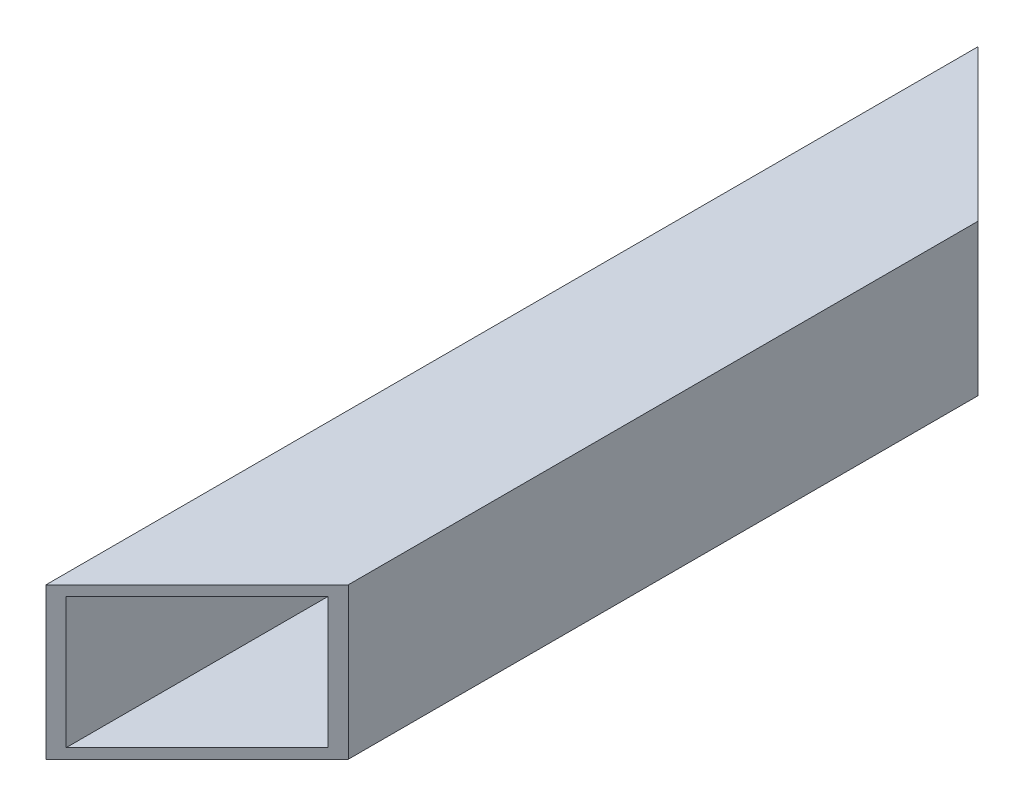
SolidWorks part; units mm, degrees
ref_plane "前视基准面" through (0, 0, 0) normal (0, 0, 1) x (1, 0, 0)
ref_plane "上视基准面" through (0, 0, 0) normal (0, 1, 0) x (1, 0, 0)
ref_plane "右视基准面" through (0, 0, 0) normal (1, 0, 0) x (0, 0, -1)
sketch "草图1" plane through (0, 0, 0) normal (0, 0, 1) x (1, 0, 0)
  line L0 (13, 13) -> (-13, 13)
  line L1 (15, -15) -> (-15, -15)
  line L2 (15, -15) -> (15, 15)
  line L3 (15, 15) -> (-15, 15)
  line L4 (-15, -15) -> (-15, 15)
  line L5 (15, -15) -> (-15, 15) construction
  line L6 (15, 15) -> (-15, -15) construction
  line L7 (-13, -13) -> (-13, 13)
  line L8 (13, -13) -> (-13, -13)
  line L9 (13, -13) -> (13, 13)
  point P0 (0, 0)
  dimension "D1" = 30
  dimension "D2" = 2
extrude "凸台-拉伸1" add sketch "草图1" along normal mid plane 185
sketch "草图2" plane through (0, 15, 0) normal (0, 1, 0) x (1, 0, 0)
  line L0 (-15, 92.5) -> (15, 62.5)
  line L1 (15, -92.5) -> (15, 92.5) construction
  line L2 (15, -62.5) -> (-15, -92.5)
  line L3 (-15, -92.5) -> (-15, 92.5) construction
  line L8 (15, 92.5) -> (-15, 92.5)
  line L9 (-15, 92.5) -> (-15, -92.5)
  line L10 (-15, -92.5) -> (15, -92.5)
  line L11 (15, -92.5) -> (15, 92.5)
  line L12 (15, 92.5) -> (-15, 92.5)
  line L13 (-15, 92.5) -> (-15, -92.5)
  line L14 (-15, -92.5) -> (15, -92.5)
  line L15 (15, -92.5) -> (15, 92.5)
  line M6 (15, 92.5) -> (-15, 92.5)
  line M8 (-15, -92.5) -> (15, -92.5)
  line M9 (15, -92.5) -> (15, 92.5)
  dimension "D1" = 0
  dimension "D2" = 45
extrude "切除-拉伸1" cut sketch "草图2" against normal blind 87 contours L2 M9 M8 | L0 M6 M9
